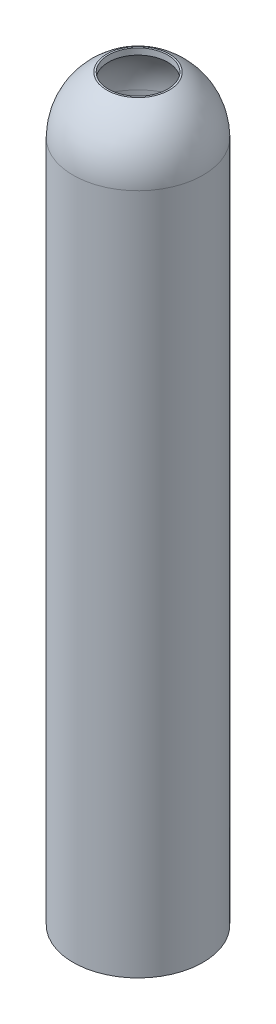
SolidWorks part; units mm, degrees
material "铁"
ref_plane "Front Plane" through (0, 0, 0) normal (0, 0, 1) x (1, 0, 0)
ref_plane "Top Plane" through (0, 0, 0) normal (0, 1, 0) x (1, 0, 0)
ref_plane "Right Plane" through (0, 0, 0) normal (1, 0, 0) x (0, 0, -1)
sketch "Sketch1" plane through (0, 0, 0) normal (0, 0, 1) x (1, 0, 0)
  line L0 (0, 0) -> (0, 25.3635) construction
  line L1 (-2.18, 0) -> (-2.18, 22.8895)
  line L2 (-1.05, 24.8) -> (-0.9946, 24.8)
  line L3 (-1.97, 0) -> (-1.97, 22.8895)
  line L5 (-2.18, 0) -> (-1.97, 0)
  line L7 (-0.9946, 24.59) -> (-0.9946, 24.8)
  line L9 (0, 24.8) -> (-1.05, 24.8) construction
  line L10 (0, 24.59) -> (-0.9946, 24.59) construction
  arc A0 (-2.18, 22.8895) -> (-1.05, 24.8) centre (0, 22.8895) cw
  arc A1 (-1.97, 22.8895) -> (-0.9946, 24.59) centre (0, 22.8895) cw
  arc A2 (-2.18, 22.8895) -> (-1.05, 24.8) centre (0, 22.8895) cw construction
  dimension "D2" = 2.18
  dimension "D1" = 4.36
  dimension "D5" = 0.21
revolve "Revolve1" add sketch "Sketch1" angle 360 about L0
